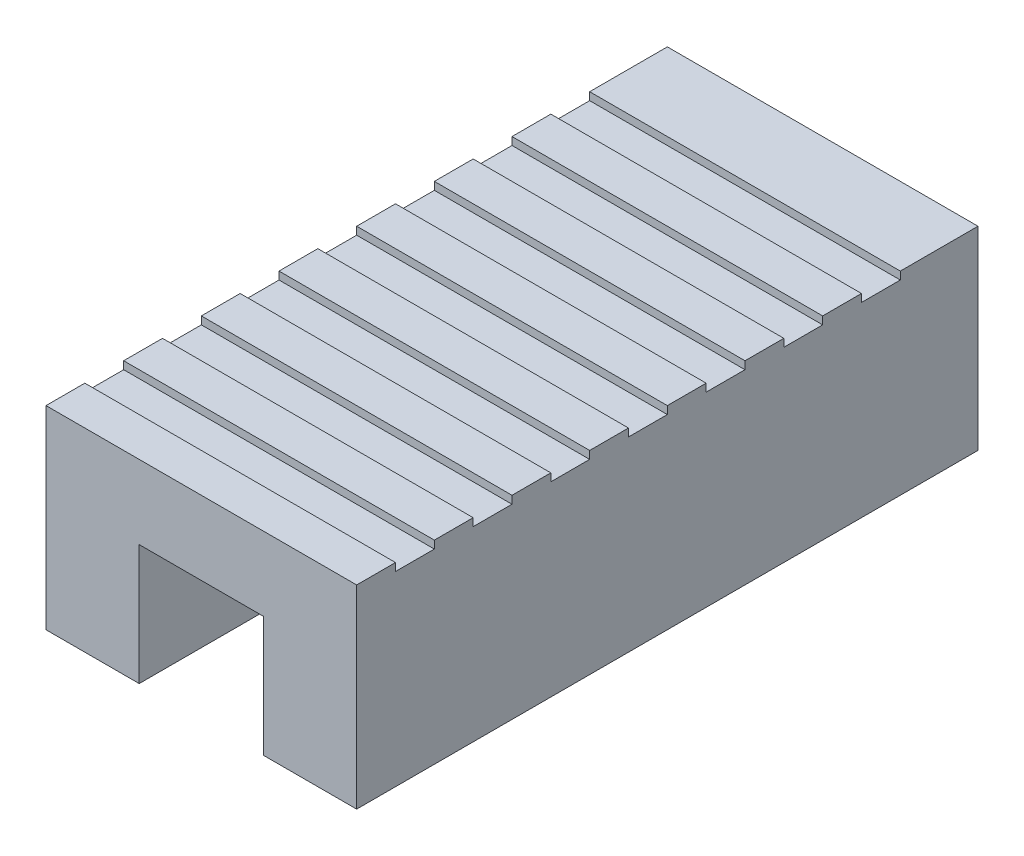
from build123d import *

# Parameters (mm, degrees)
BOSS_EXTRUDE1_DEPTH = 160
SKETCH2_W           = 80
SKETCH2_H           = 10
CUT_EXTRUDE1_DEPTH  = 2
LPATTERN1_COUNT     = 8
LPATTERN1_PITCH     = 20


with BuildPart() as part:
    # Sketch1 → Boss-Extrude1 (new body)
    with BuildSketch(Plane.XY):
        Polygon((0, 6), (0, 25), (-40, 25), (-40, -25), (-16, -25), (-16, 6), align=None)
        Polygon((40, 25), (0, 25), (0, 6), (16, 6), (16, -25), (40, -25), align=None)
    extrude(amount=BOSS_EXTRUDE1_DEPTH)

    # Sketch2 → Cut-Extrude1 (cut)
    with BuildSketch(Plane(origin=(0, 25, 0), x_dir=(1, 0, 0), z_dir=(0, 1, 0))):
        with Locations((0, -25)):
            Rectangle(SKETCH2_W, SKETCH2_H)
    cut_extrude1 = extrude(amount=-CUT_EXTRUDE1_DEPTH, mode=Mode.SUBTRACT)

    # LPattern1: Cut-Extrude1 ×8
    with Locations(*[(0, 0, i * LPATTERN1_PITCH) for i in range(1, LPATTERN1_COUNT)]):
        add(cut_extrude1, mode=Mode.SUBTRACT)


solid = part.part
